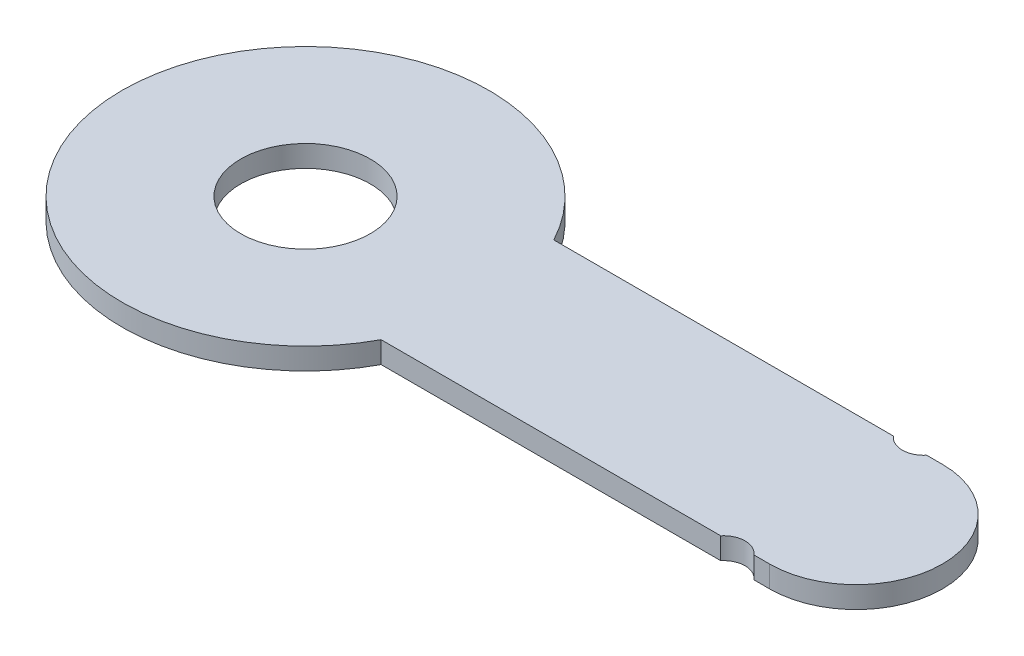
from build123d import *

# Parameters (mm, degrees)
SKETCH1_R           = 1.5
BOSS_EXTRUDE1_DEPTH = 0.5
SKETCH2_R           = 0.5
CUT_EXTRUDE1_DEPTH  = 16.358222553


with BuildPart() as part:
    # Sketch1 → Boss-Extrude1 (new body)
    with BuildSketch(Plane(origin=(0, 0, 0), x_dir=(1, 0, 0), z_dir=(0, 1, 0))):
        with BuildLine():
            Line((12.75, 2), (3.75, 2))
            ThreePointArc((3.75, 2), (-4.25, 0), (3.75, -2))
            Line((3.75, -2), (12.75, -2))
            ThreePointArc((12.75, -2), (14.75, 0), (12.75, 2))
        make_face()
        with Locations(Location((0, 0, 0), (0, 0, 270))):
            Circle(SKETCH1_R, mode=Mode.SUBTRACT)
    extrude(amount=BOSS_EXTRUDE1_DEPTH)

    # Sketch2 → Cut-Extrude1 (cut, through all)
    with BuildSketch(Plane(origin=(0, 0.5, 0), x_dir=(1, 0, 0), z_dir=(0, 1, 0))):
        with Locations((12, 2.32)):
            Circle(SKETCH2_R)
        with Locations((12, -2.32)):
            Circle(SKETCH2_R)
    extrude(amount=-CUT_EXTRUDE1_DEPTH, mode=Mode.SUBTRACT)


solid = part.part
